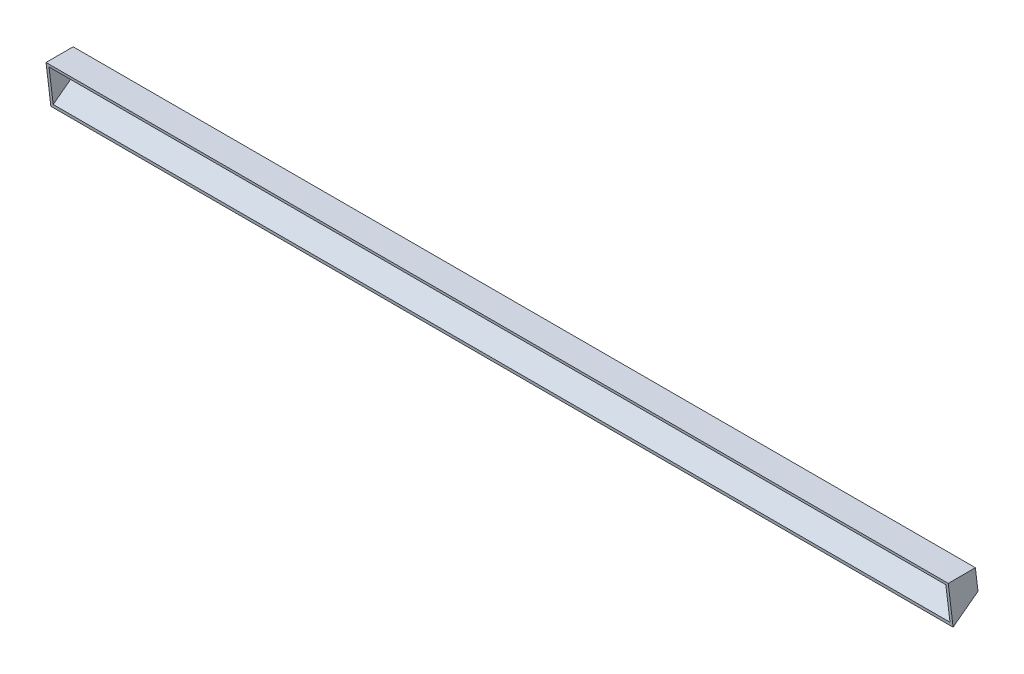
from build123d import *

# Parameters (mm, degrees)
BOSS_EXTRUDE1_DEPTH = 2
BOSS_EXTRUDE2_DEPTH = 661
BOSS_EXTRUDE3_DEPTH = 2


with BuildPart() as part:
    # Sketch1 → Boss-Extrude1 (new body)
    with BuildSketch(Plane(origin=(0, 0, 0), x_dir=(0, 0, -1), z_dir=(1, 0, 0))):
        Polygon((0, 0), (-20, 0), (-16.414240878, -29.78493464), (1.929767975, -16.029524307), align=None)
    extrude(amount=BOSS_EXTRUDE1_DEPTH)

    # Sketch2 → Boss-Extrude2 (add)
    with BuildSketch(Plane.ZY):
        Polygon((0, 0), (20, 0), (19.759223301, -2), (1.773664518, -2), (0.193910267, -15.122152246), (16.690272744, -27.492089303), (16.414240878, -29.78493464), (-1.929767975, -16.029524307), align=None)
    extrude(amount=BOSS_EXTRUDE2_DEPTH)

    # Sketch3 → Boss-Extrude3 (add)
    with BuildSketch(Plane.ZY.offset(661)):
        Polygon((20, 0), (0, 0), (-1.929767975, -16.029524307), (16.414240878, -29.78493464), align=None)
    extrude(amount=BOSS_EXTRUDE3_DEPTH)


solid = part.part
